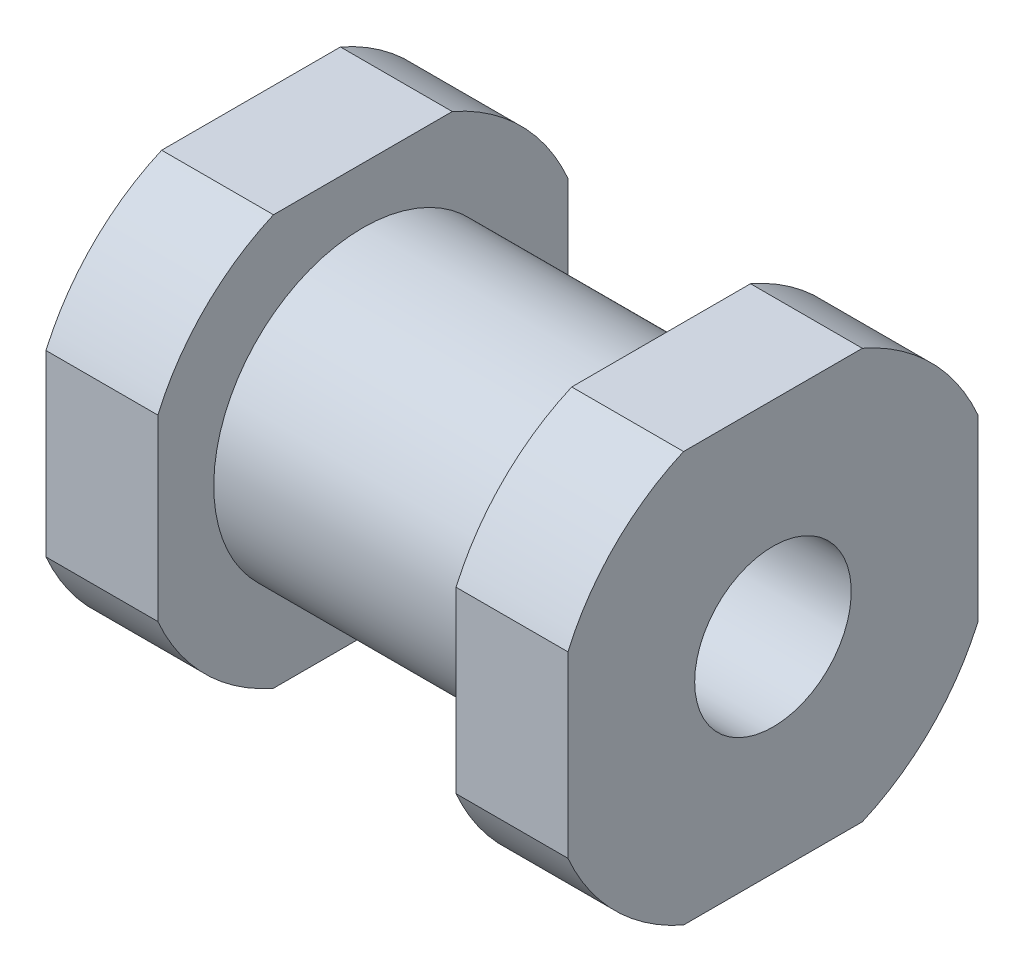
SolidWorks part; units mm, degrees
material "S45C"
ref_plane "Front Plane" through (0, 0, 0) normal (0, 0, 1) x (1, 0, 0)
ref_plane "Top Plane" through (0, 0, 0) normal (0, 1, 0) x (1, 0, 0)
ref_plane "Right Plane" through (0, 0, 0) normal (1, 0, 0) x (0, 0, -1)
sketch "Sketch1" plane through (0, 0, 0) normal (0, 0, 1) x (1, 0, 0)
  line L0 (0, 6) -> (0, 0)
  line L1 (0, 6) -> (3, 6)
  line L2 (3, 6) -> (3, 4)
  line L3 (3, 4) -> (11, 4)
  line L4 (11, 4) -> (11, 6)
  line L5 (11, 6) -> (14, 6)
  line L6 (14, 6) -> (14, 0)
  line L7 (14, 0) -> (0, 0) construction
  line L8 (0, 0) -> (14, 0)
  dimension "D1" = 8
  dimension "D2" = 12
  dimension "D3" = 3
  dimension "D4" = 3
  dimension "D5" = 14
revolve "Revolve1" add sketch "Sketch1" angle 360 about L7
hole_wizard "M5 Tapped Hole1" positions "Sketch3" profile "Sketch2" tap size "M5" standard "GB" end condition through all
sketch "Sketch3" plane through (0, 0, 0) normal (-1, 0, 0) x (0, 0, 1)
  point P0 (0, 0)
cosmetic thread "Cosmetic Thread 1" parameters "D2"=5
sketch "Sketch2" plane through (0, 0, 0) normal (0, 1, 0) x (0, 0, 1)
  line L0 (0, 0) -> (0, 14)
  line L1 (0, 14) -> (2.1, 14)
  line L2 (2.1, 14) -> (2.1, 0)
  line L5 (2.1, 0) -> (0, 0)
  line L11 (0, -6.35) -> (0, 107.95) construction
  dimension "通孔螺纹孔钻头直径" = 4.2
  dimension "通孔螺纹孔钻头深度" = 14
sketch "Sketch4" plane through (0, 0, 0) normal (-1, 0, 0) x (0, 0, 1)
  line L1 (-5.5, -5.5) -> (5.5, -5.5)
  line L2 (-5.5, -5.5) -> (-5.5, 5.5)
  line L3 (-5.5, 5.5) -> (5.5, 5.5)
  line L4 (5.5, -5.5) -> (5.5, 5.5)
  line L5 (-5.5, -5.5) -> (5.5, 5.5) construction
  line L6 (-5.5, 5.5) -> (5.5, -5.5) construction
  point P0 (0, 0)
  dimension "D1" = 11
  dimension "D2" = 11
extrude "Cut-Extrude1" cut sketch "Sketch4" against normal through all flip side to cut
